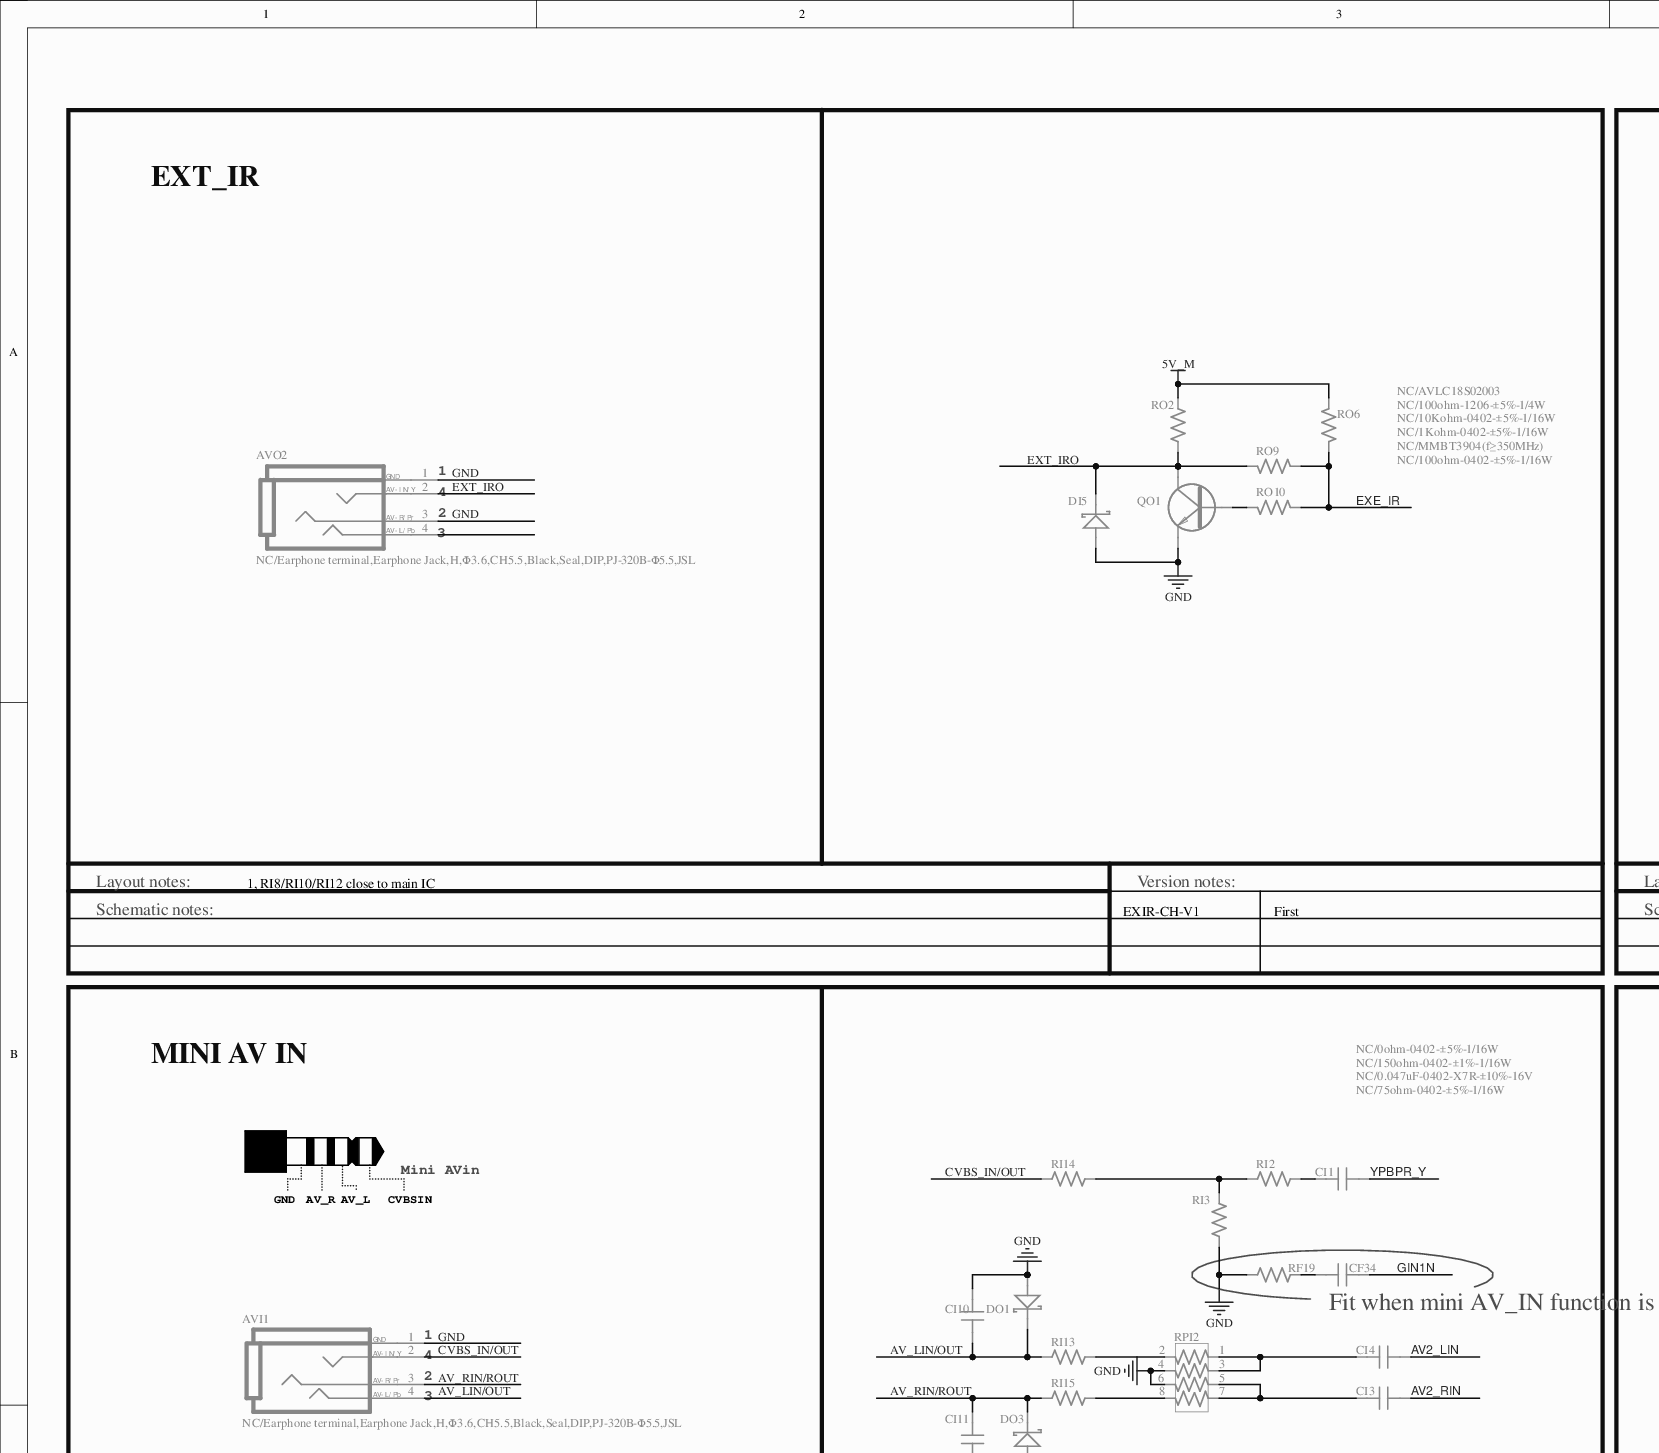
[diagram p0: MISC84438-10.SchDoc, top left]
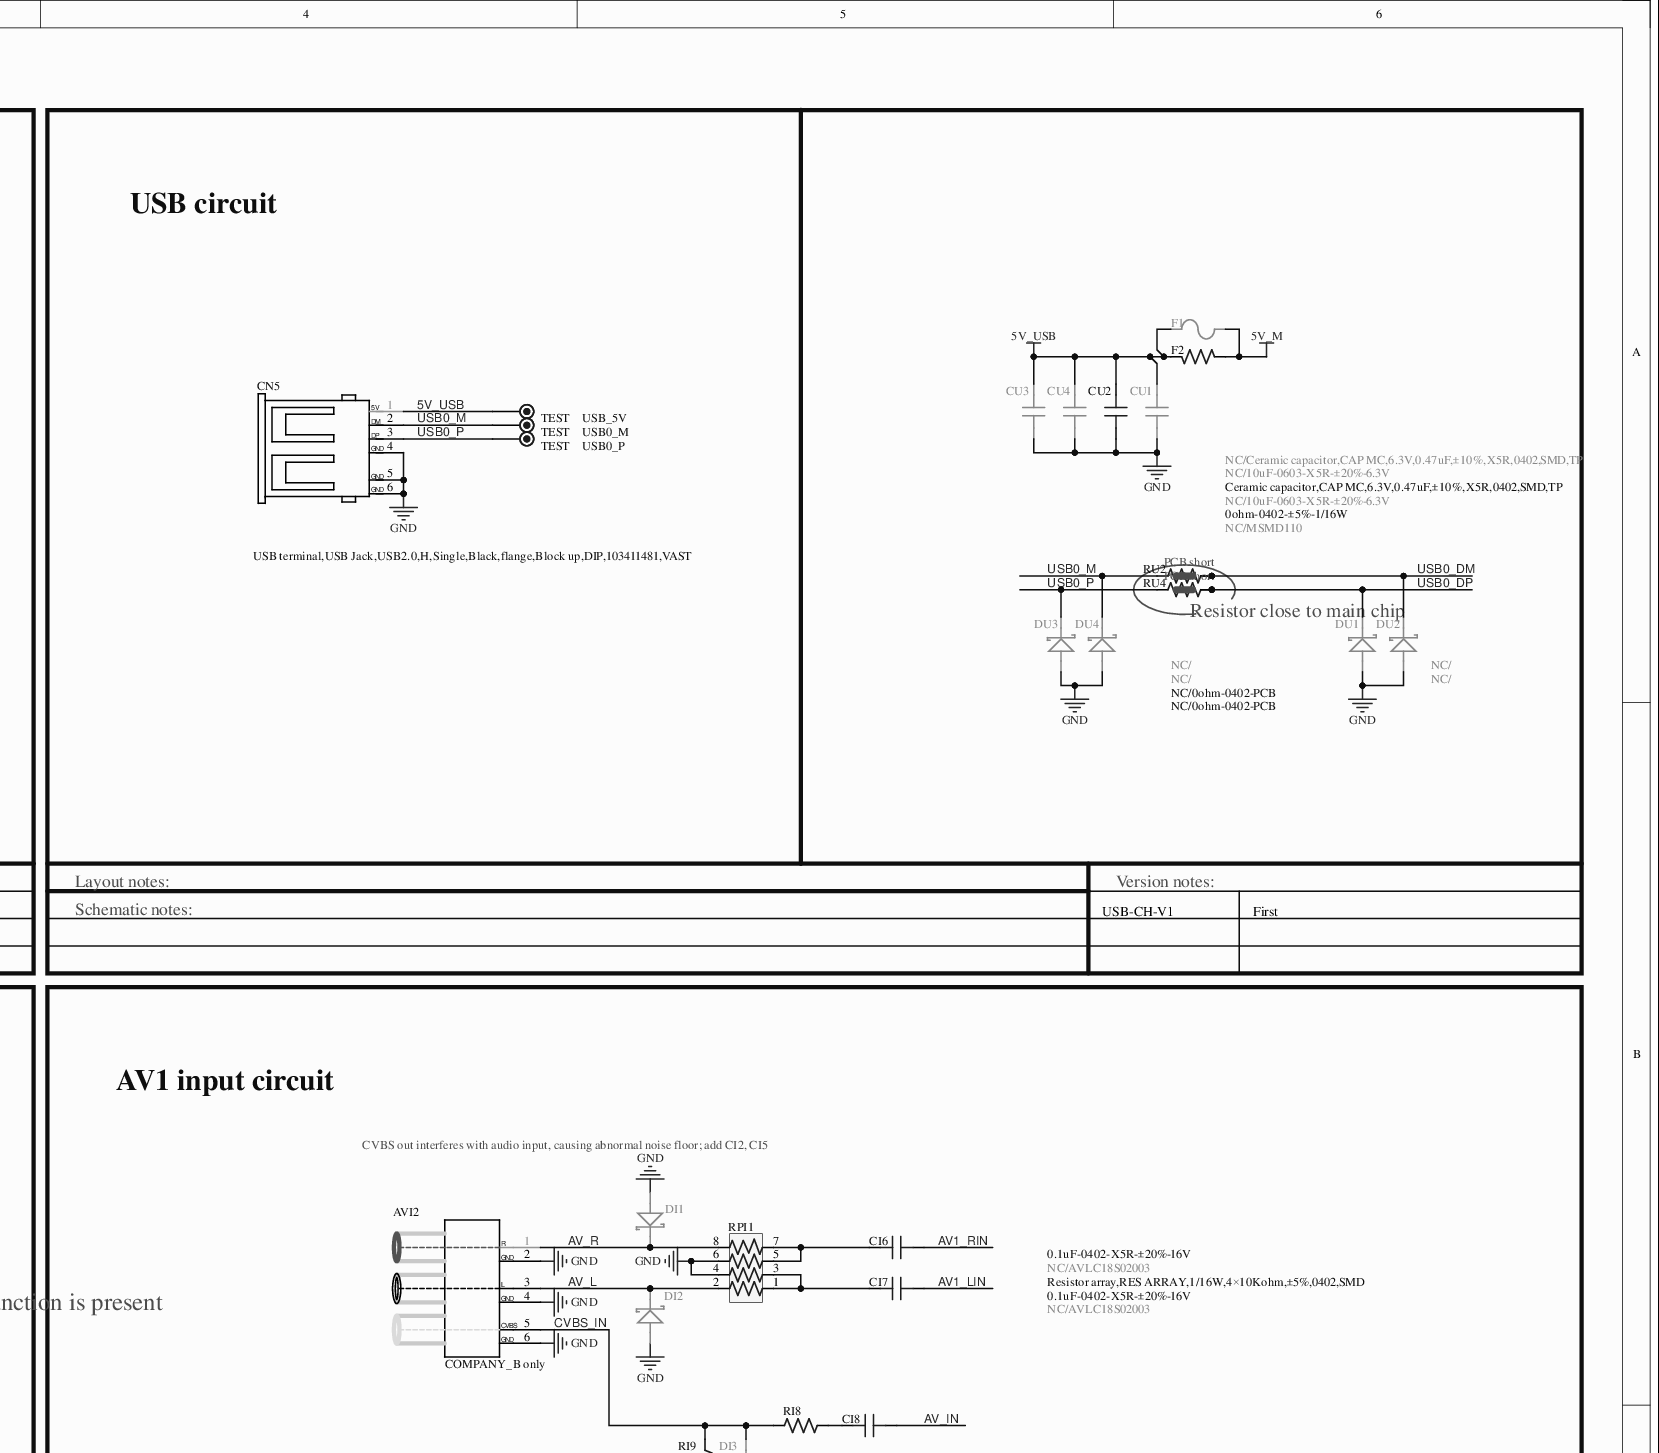
[diagram p1: MISC84438-10.SchDoc, top right]
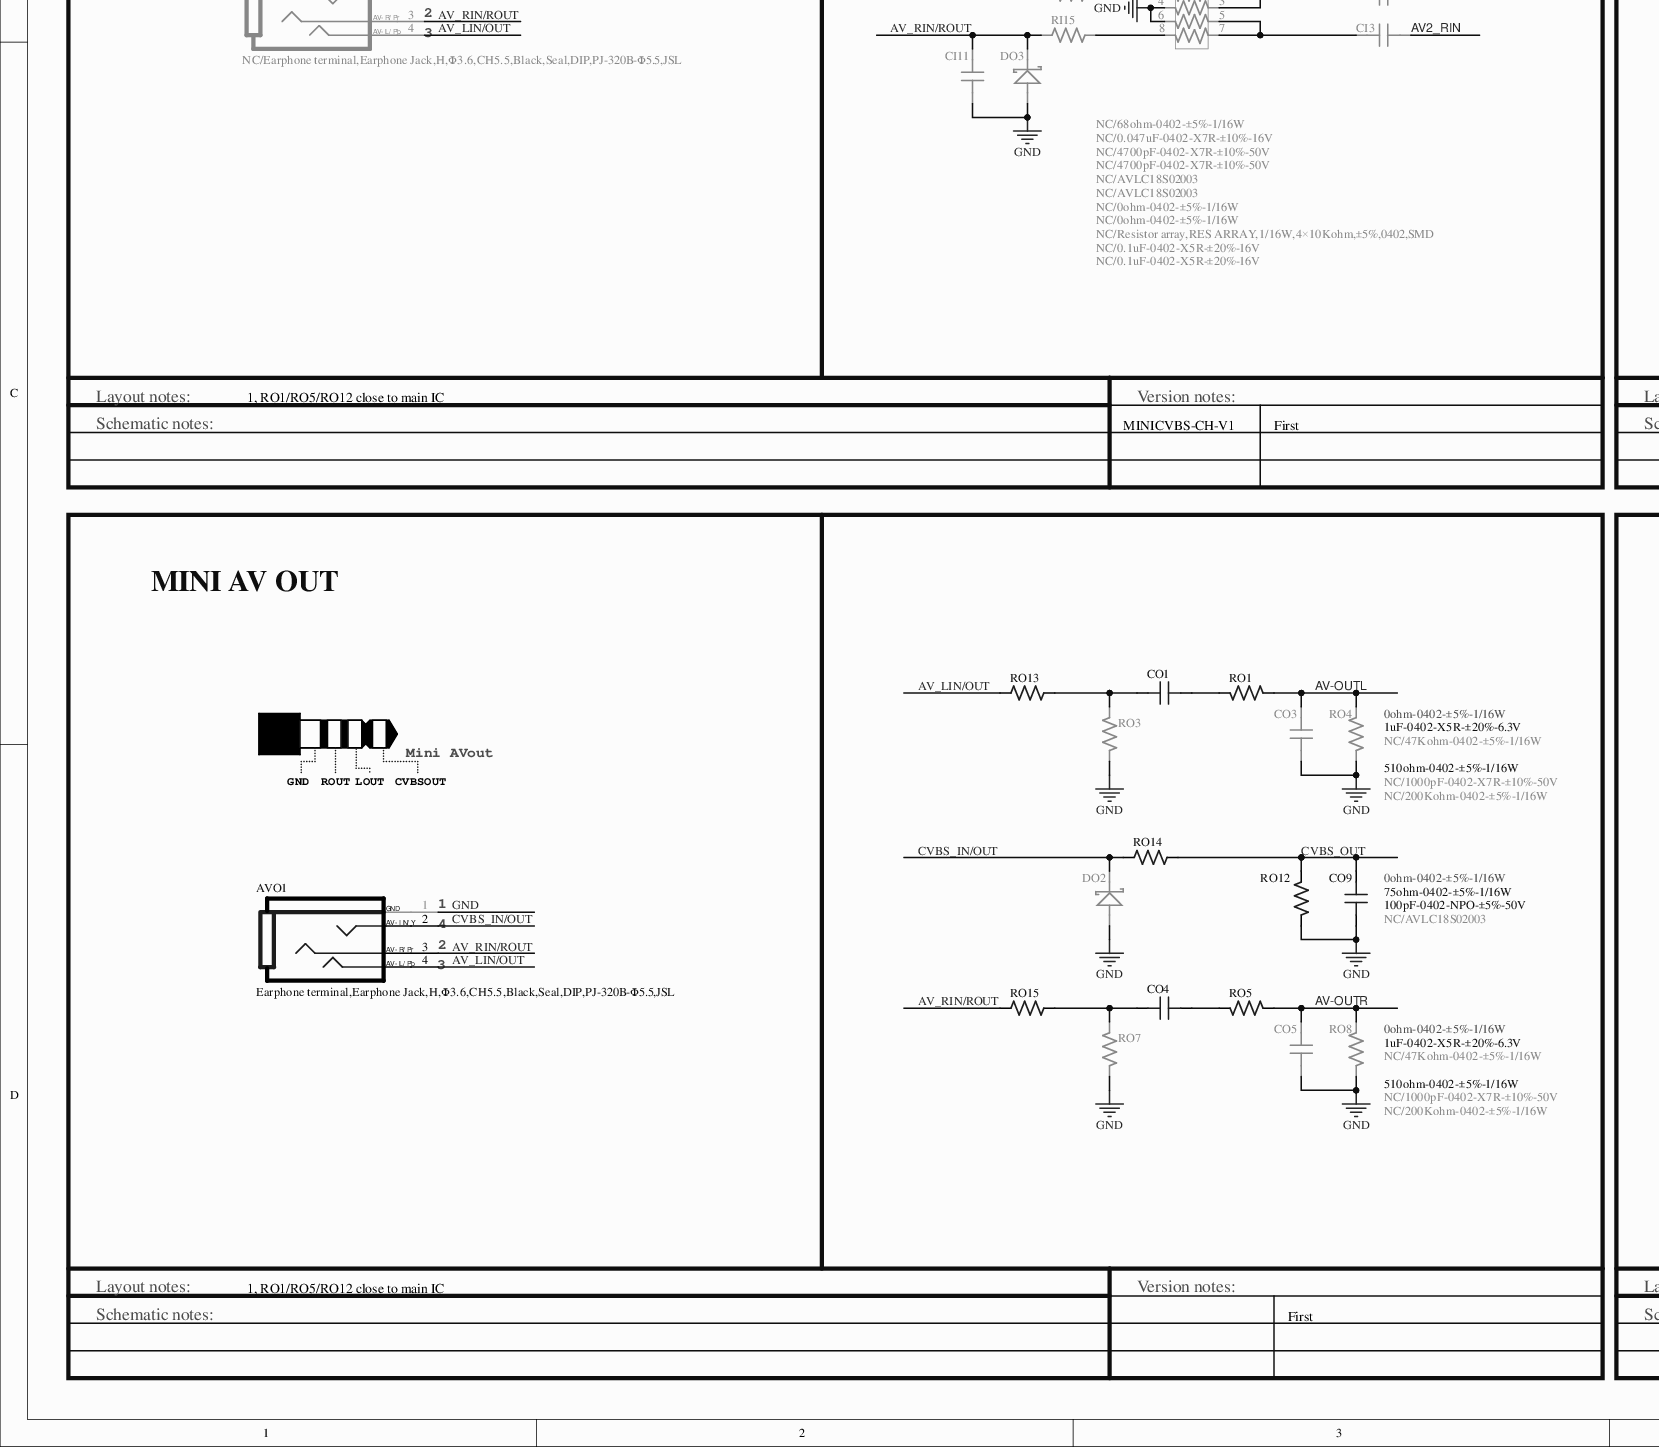
[diagram p2: MISC84438-10.SchDoc, bottom left]
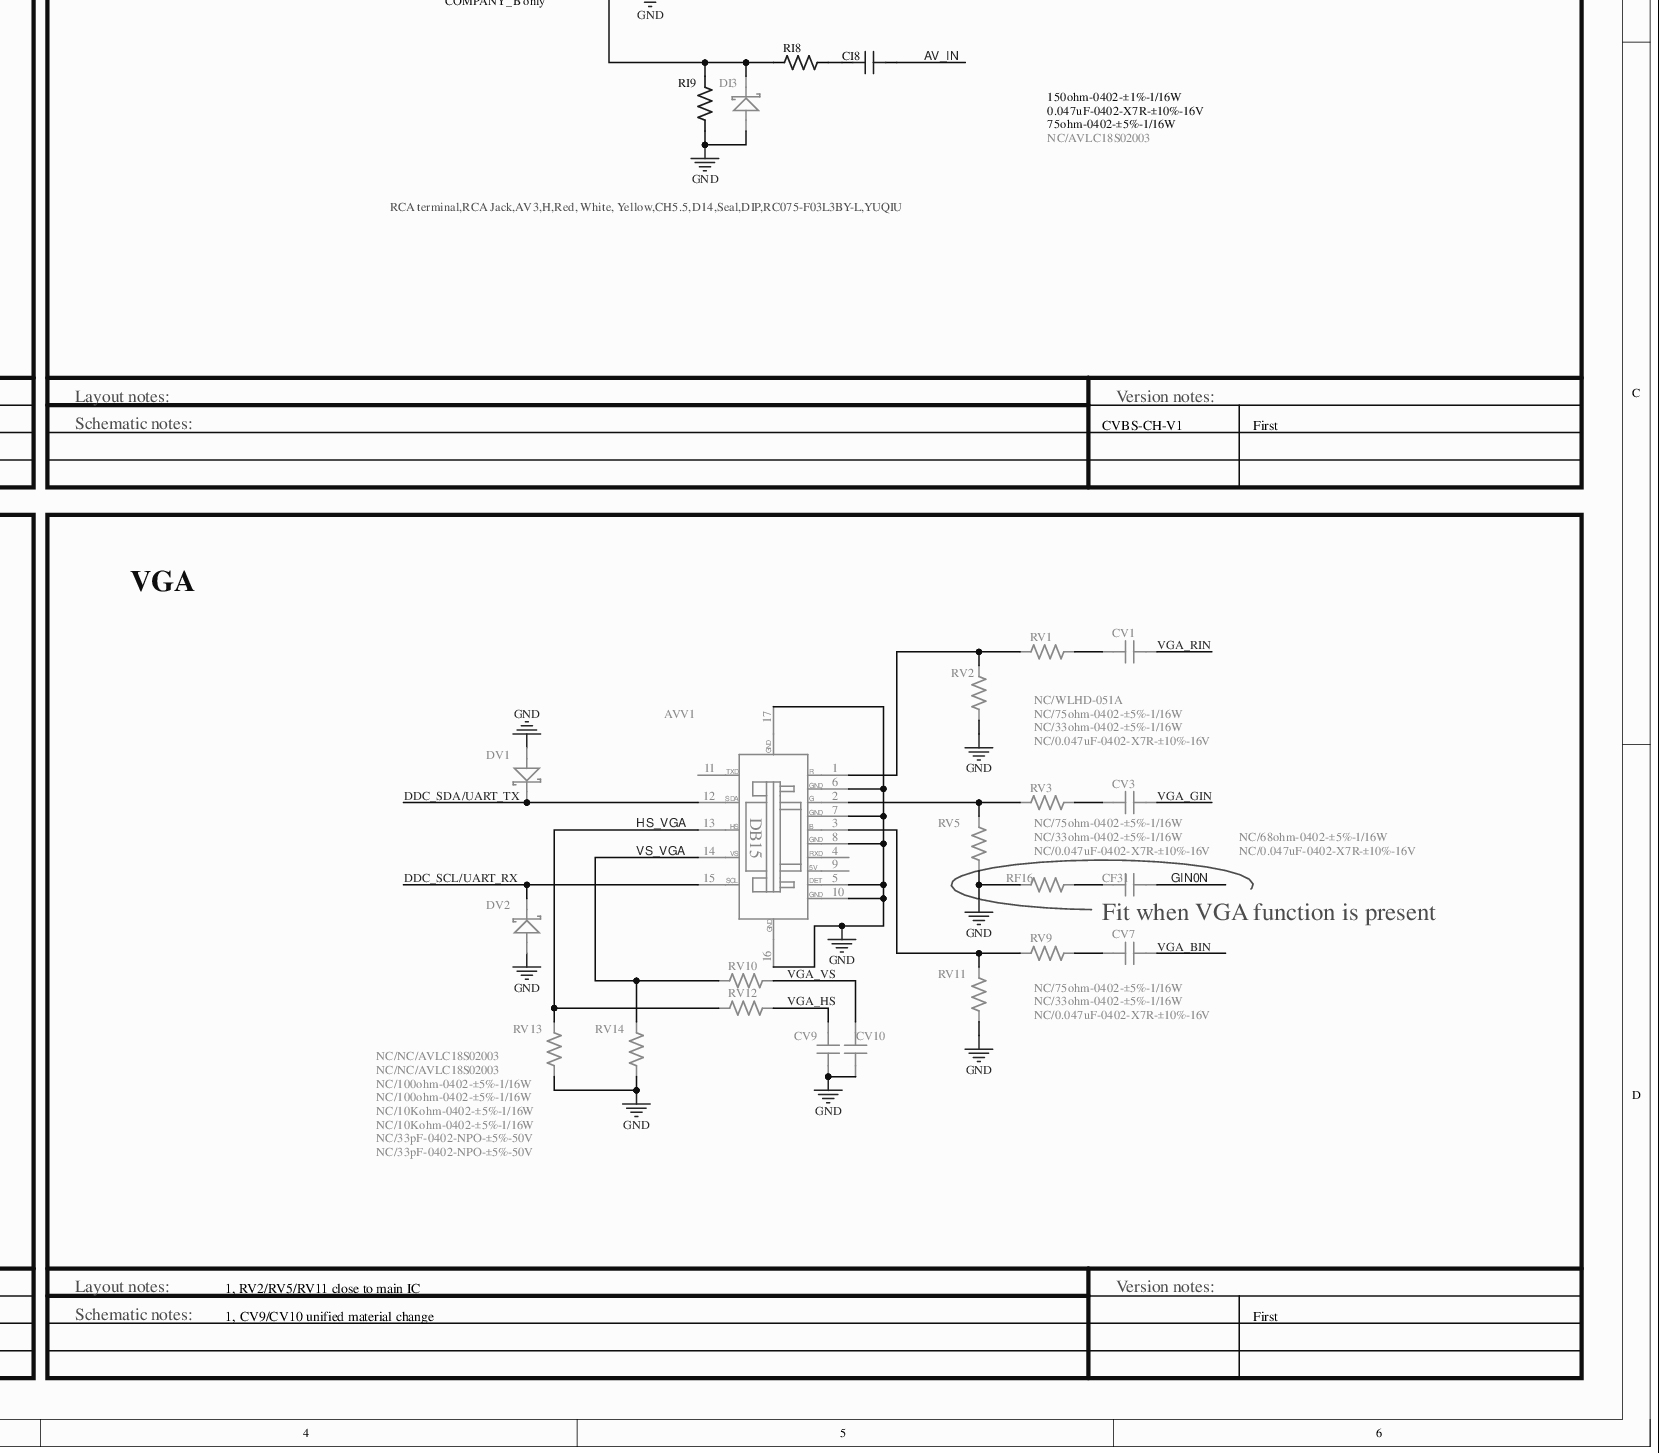
[diagram p3: MISC84438-10.SchDoc, bottom right]
# Altium project MISC84438-18.PrjPCB (part 5 of 8)

## Sheet MISC84438-10.SchDoc
size 596 x 520 mm

### Parts
AVI1  NC/Earphone terminal,Earphone Jack,H,Φ3.6,CH5.5,Black,Seal,DIP,PJ-320B-Φ5.5,JSL  [PHONE-HD-43]
AVI2  RCA terminal,RCA Jack,AV3,H,Red, White, Yellow,CH5.5,D14,Seal,DIP,RC075-F03L3BY-L,YUQIU  [AV3-H14-15]
AVO1  Earphone terminal,Earphone Jack,H,Φ3.6,CH5.5,Black,Seal,DIP,PJ-320B-Φ5.5,JSL  [PHONE-HD-43]
AVO2  NC/Earphone terminal,Earphone Jack,H,Φ3.6,CH5.5,Black,Seal,DIP,PJ-320B-Φ5.5,JSL  [PHONE-HD-43]
AVV1  NC/WLHD-051A  [DB15-HF-1]
CF31  NC/0.047uF-0402-X7R-±10%-16V  [C0402]
CF34  NC/0.047uF-0402-X7R-±10%-16V  [C0402]
CI1  NC/0.047uF-0402-X7R-±10%-16V  [C0402]
CI3  NC/0.1uF-0402-X5R-±20%-16V  [C0402]
CI4  NC/0.1uF-0402-X5R-±20%-16V  [C0402]
CI6  0.1uF-0402-X5R-±20%-16V  [C0402]
CI7  0.1uF-0402-X5R-±20%-16V  [C0402]
CI8  0.047uF-0402-X7R-±10%-16V  [C0402]
CI10  NC/4700pF-0402-X7R-±10%-50V  [C0402]
CI11  NC/4700pF-0402-X7R-±10%-50V  [C0402]
CN5  USB terminal,USB Jack,USB2.0,H,Single,Black,flange,Block up,DIP,103411481,VAST  [USB-HD-30]
CO1  1uF-0402-X5R-±20%-6.3V  [C0402]
CO3  NC/1000pF-0402-X7R-±10%-50V  [C0402]
CO4  1uF-0402-X5R-±20%-6.3V  [C0402]
CO5  NC/1000pF-0402-X7R-±10%-50V  [C0402]
CO9  100pF-0402-NPO-±5%-50V  [C0402]
CU1  NC/10uF-0603-X5R-±20%-6.3V  [C0603]
CU2  Ceramic capacitor,CAP MC,6.3V,0.47uF,±10%,X5R,0402,SMD,TP  [C0402]
CU3  NC/Ceramic capacitor,CAP MC,6.3V,0.47uF,±10%,X5R,0402,SMD,TP  [C0402]
CU4  NC/10uF-0603-X5R-±20%-6.3V  [C0603]
CV1  NC/0.047uF-0402-X7R-±10%-16V  [C0402]
CV3  NC/0.047uF-0402-X7R-±10%-16V  [C0402]
CV7  NC/0.047uF-0402-X7R-±10%-16V  [C0402]
CV9  NC/33pF-0402-NPO-±5%-50V  [C0402]
CV10  NC/33pF-0402-NPO-±5%-50V  [C0402]
DI1  NC/AVLC18S02003  [DIODE-S0402]
DI2  NC/AVLC18S02003  [DIODE-S0402]
DI3  NC/AVLC18S02003  [DIODE-S0402]
DI5  NC/AVLC18S02003  [DIODE-S0402]
DO1  NC/AVLC18S02003  [DIODE-S0402]
DO2  NC/AVLC18S02003  [DIODE-S0402]
DO3  NC/AVLC18S02003  [DIODE-S0402]
DU1  NC/  [DIODE-S0402]
DU2  NC/  [DIODE-S0402]
DU3  NC/  [DIODE-S0402]
DU4  NC/  [DIODE-S0402]
DV1  NC/NC/AVLC18S02003  [DIODE-S0402]
DV2  NC/NC/AVLC18S02003  [DIODE-S0402]
F1  NC/MSMD110  [FUSE3.5A-S]
F2  0ohm-0402-±5%-1/16W  [R0402]
QO1  NC/MMBT3904(f≥350MHz)  [SOT-23]
RF16  NC/68ohm-0402-±5%-1/16W  [R0402]
RF19  NC/68ohm-0402-±5%-1/16W  [R0402]
RI2  NC/150ohm-0402-±1%-1/16W  [R0402]
RI3  NC/75ohm-0402-±5%-1/16W  [R0402]
RI8  150ohm-0402-±1%-1/16W  [R0402]
RI9  75ohm-0402-±5%-1/16W  [R0402]
RI13  NC/0ohm-0402-±5%-1/16W  [R0402]
RI14  NC/0ohm-0402-±5%-1/16W  [R0402]
RI15  NC/0ohm-0402-±5%-1/16W  [R0402]
RO1  510ohm-0402-±5%-1/16W  [R0402]
RO2  NC/100ohm-1206-±5%-1/4W  [R1206]
RO3  NC/47Kohm-0402-±5%-1/16W  [R0402]
RO4  NC/200Kohm-0402-±5%-1/16W  [R0402]
RO5  510ohm-0402-±5%-1/16W  [R0402]
RO6  NC/10Kohm-0402-±5%-1/16W  [R0402]
RO7  NC/47Kohm-0402-±5%-1/16W  [R0402]
RO8  NC/200Kohm-0402-±5%-1/16W  [R0402]
RO9  NC/100ohm-0402-±5%-1/16W  [R0402]
RO10  NC/1Kohm-0402-±5%-1/16W  [R0402]
RO12  75ohm-0402-±5%-1/16W  [R0402]
RO13  0ohm-0402-±5%-1/16W  [R0402]
RO14  0ohm-0402-±5%-1/16W  [R0402]
RO15  0ohm-0402-±5%-1/16W  [R0402]
RPI1  Resistor array,RES ARRAY,1/16W,4×10Kohm,±5%,0402,SMD  [RA0402]
RPI2  NC/Resistor array,RES ARRAY,1/16W,4×10Kohm,±5%,0402,SMD  [RA0402]
RU2  NC/0ohm-0402-PCB  [R0402SC]
RU4  NC/0ohm-0402-PCB  [R0402SC]
RV1  NC/33ohm-0402-±5%-1/16W  [R0402]
RV2  NC/75ohm-0402-±5%-1/16W  [R0402]
RV3  NC/33ohm-0402-±5%-1/16W  [R0402]
RV5  NC/75ohm-0402-±5%-1/16W  [R0402]
RV9  NC/33ohm-0402-±5%-1/16W  [R0402]
RV10  NC/100ohm-0402-±5%-1/16W  [R0402]
RV11  NC/75ohm-0402-±5%-1/16W  [R0402]
RV12  NC/100ohm-0402-±5%-1/16W  [R0402]
RV13  NC/10Kohm-0402-±5%-1/16W  [R0402]
RV14  NC/10Kohm-0402-±5%-1/16W  [R0402]
USB0_M  TEST  [TP]
USB0_P  TEST  [TP]
USB_5V  TEST  [TP]

### Blocks framed on the sheet
EXT_IR: AVO2 DI5 QO1 RO2 RO6 RO9 RO10
USB circuit: CN5 CU1-CU4 DU1-DU4 F1 F2 RU2 RU4 USB0_M USB0_P USB_5V
MINI AV IN: AVI1 CF34 CI1 CI3 CI4 CI10 CI11 DO1 DO3 RF19 RI2 RI3 RI13-RI15 RPI2
AV1 input circuit: AVI2 CI6-CI8 DI1-DI3 RI8 RI9 RPI1
MINI AV OUT: AVO1 CO1 CO3-CO5 CO9 DO2 RO1 RO3-RO5 RO7 RO8 RO12-RO15
VGA: AVV1 CF31 CV1 CV3 CV7 CV9 CV10 DV1 DV2 RF16 RV1-RV3 RV5 RV9-RV14

### Nets
5V_M: F1.2 F2.1 RO2.2 RO6.1
5V_USB: CN5.1 CU1.2 CU2.1 CU3.1 CU4.2 F1.1 F2.2 USB_5V.1
GND: AVI1.1 AVI2.2(GND) AVI2.4(GND) AVI2.6(GND) AVO1.1 AVO2.1 AVO2.3 AVV1.5 AVV1.6(GND) AVV1.7(GND) AVV1.8(GND) AVV1.10(GND) AVV1.16(Shell) AVV1.17(Shell) CI10.2 CI11.2 CN5.4 CN5.5 CN5.6 CO3.1 CO5.1 CO9.1 CU1.1 CU2.2 CU3.2 CU4.1 CV9.1 CV10.1 DI1.A DI2.A DI3.A DI5.A DO1.A DO2.A DO3.A DU1.A DU2.A DU3.A DU4.A DV1.A DV2.A QO1.E RF16.2 RF19.1 RI3.1 RI9.1 RO3.1 RO4.1 RO7.1 RO8.1 RO12.2 RPI1.4 RPI1.6 RPI2.4 RPI2.6 RV2.1 RV5.1 RV11.1 RV13.2 RV14.2
AV1_LIN: CI7.1
AV1_RIN: CI6.1
AV2_LIN: CI4.1
AV2_RIN: CI3.1
AV-OUTL: CO3.2 RO1.1 RO4.2
AV-OUTR: CO5.2 RO5.1 RO8.2
AV_IN: CI8.1
AV_L: AVI2.3(Rin) DI2.K RPI1.2
AV_LIN/OUT: AVI1.4 AVO1.4 CI10.1 DO1.K RI13.1 RO13.1
AV_R: AVI2.1(Lin) DI1.K RPI1.8
AV_RIN/ROUT: AVI1.3 AVO1.3 CI11.1 DO3.K RI15.1 RO15.1
CVBS_IN: AVI2.5(CVBS) DI3.K RI8.1 RI9.2
CVBS_IN/OUT: AVI1.2 AVO1.2 DO2.K RI14.1 RO14.1
CVBS_OUT: CO9.2 RO12.1 RO14.2
DDC_SCL/UART_RX: AVV1.15(SCL) DV2.K
DDC_SDA/UART_TX: AVV1.12(SDA) DV1.K
EXE_IR: RO6.2 RO9.2 RO10.2
EXT_IRO: AVO2.2 DI5.K QO1.C RO2.1 RO9.1
GIN0N: CF31.1
GIN1N: CF34.2
HS_VGA: AVV1.13(HS) RV12.1 RV13.1
USB0_DM: DU2.K RU2.2 RU2.3
USB0_DP: DU1.K RU4.2 RU4.3
USB0_M: CN5.2 DU4.K RU2.1 USB0_M.1
USB0_P: CN5.3 DU3.K RU4.1 USB0_P.1
VGA_BIN: CV7.1
VGA_GIN: CV3.1
VGA_HS: CV9.2 RV12.2
VGA_RIN: CV1.1
VGA_VS: CV10.2 RV10.2
VS_VGA: AVV1.14(VS) RV10.1 RV14.1
YPBPR_Y: CI1.1
NetAVV1_1: AVV1.1(R) RV1.2 RV2.2
NetAVV1_2: AVV1.2(G) RV3.2 RV5.2
NetAVV1_3: AVV1.3(B) RV9.2 RV11.2
NetCF31_2: CF31.2 RF16.1
NetCF34_1: CF34.1 RF19.2
NetCI1_2: CI1.2 RI2.2
NetCI3_2: CI3.2 RPI2.5 RPI2.7
NetCI4_2: CI4.2 RPI2.1 RPI2.3
NetCI6_2: CI6.2 RPI1.5 RPI1.7
NetCI7_2: CI7.2 RPI1.1 RPI1.3
NetCI8_2: CI8.2 RI8.2
NetCO1_1: CO1.1 RO3.2 RO13.2
NetCO1_2: CO1.2 RO1.2
NetCO4_1: CO4.1 RO7.2 RO15.2
NetCO4_2: CO4.2 RO5.2
NetCV1_2: CV1.2 RV1.1
NetCV3_2: CV3.2 RV3.1
NetCV7_2: CV7.2 RV9.1
NetQO1_B: QO1.B RO10.1
NetRI2_1: RI2.1 RI3.2 RI14.2
NetRI13_2: RI13.2 RPI2.2
NetRI15_2: RI15.2 RPI2.8

Not connected (* = marked no-connect by the designer): AVO2 4*; AVV1 4(NC)* 9(NC)* 11(NC)*

### Notes on the sheet
- (near AVO2) 4
- (near AVO2) 1
- (near AVO2) 2
- (near AVO2) 3
- Resistor close to main chip
- Layout notes:
- Schematic notes:
- 1, RI8/RI10/RI12 close to main IC
- EXIR-CH-V1
- Version notes:
- First
- USB-CH-V1
- Mini AVin
- (near DI1) CVBS out interferes with audio input, causing abnormal noise floor; add CI2, CI5
- GND
- AV_R
- AV_L
- CVBSIN
- (near CF34) Fit when mini AV_IN function is present
- (near AVI1) 2
- (near AVI1) 4
- (near AVI1) 1
- (near AVI1) 3
- 1, RO1/RO5/RO12 close to main IC
- MINICVBS-CH-V1
- CVBS-CH-V1
- ROUT
- LOUT
- CVBSOUT
- Mini AVout
- (near AVO1) 4
- (near AVO1) 1
- (near CF31) Fit when VGA function is present
- (near AVO1) 2
- (near AVO1) 3
- MINIAVOUT-COMPANY_A-V1
- 1, RV2/RV5/RV11 close to main IC
- 1, CV9/CV10 unified material change
- VGA-COMPANY_A-V69D-V1

### Library data of the parts
AVI1 AVO1 AVO2 = 耳机端子,Earphone Jack,H,Φ3.6,CH5.5,Black,DIP-DLMI
AVI2 = XXX.XXX.0003577-DLMI: RCA terminal,RCA Jack,AV3,H,Red, White, Yellow,CH5.5,D14,Seal,DIP,RC075-F03L3BY-L,YUQIU-DLMI
AVV1 = WLHD-051A-DLMI-DB15: CN-DB15-horizontal-#-#-#
CF31 CF34 CI1 CI8 CV1 CV3 CV7 = 0.047uF-0402-X7R-±10%-16V-D
CI3 CI4 CI6 CI7 CU2 CU3 = 0.1uF-0402-Y5V-+80%-20%-16V-D
CI10 CI11 = 1000pF-0402-X7R-±10%-50V-D
CN5 = PKG-003212/P000071027: USB terminal,USB2.0,H,Single,Block up,DIP,U250FD004S1549BY-DLMI
CO1 CO4 = 1uF-0402-X5R-±20%-6.3V-D
CO3 CO5 CO9 = 100pF-0402-NPO-±5%-50V-D
CU1 CU4 = 10uF-0603-X5R-±20%-6.3V-D
CV9 CV10 = 30pF-0402-NPO-±5%-50V-D
DI1-DI3 DI5 DO1-DO3 DU1-DU4 DV1 DV2 = AVLC18S02003-D
F1 = MSMD110-D: FUSE
F2 = 5R1ohm-0402-±5%-1/16W-D
QO1 = LMBT3904LT1G-D-NPN: Q-NPN-#-#-#
RF16 RF19 = 68ohm-0402-±5%-1/16W-D
RI2 RI8 = 150ohm-0402-±1%-1/16W-D
RI3 RI9 RO12 RV2 RV5 RV11 = 75ohm-0402-±5%-1/16W-D
RI13-RI15 RO13-RO15 = 0ohm-0402-±5%-1/16W-D
RO1 RO5 = 510ohm-0402-±5%-1/16W-D
RO2 = 100ohm-1206-±5%-1/4W-D: RES
RO3 RO7 = 47Kohm-0402-±5%-1/16W-D
RO4 RO8 = 200Kohm-0402-±5%-1/16W-D
RO6 RV13 RV14 = 10Kohm-0402-±5%-1/16W-D
RO9 RV10 RV12 = 100ohm-0402-±5%-1/16W-D
RO10 = 1Kohm-0402-±5%-1/16W-D
RPI1 RPI2 = 4*100ohm-0402-±5%-1/16W-D
RU2 RU4 = 0ohm-0402-PCB-D
RV1 RV3 RV9 = 33ohm-0402-±5%-1/16W-D